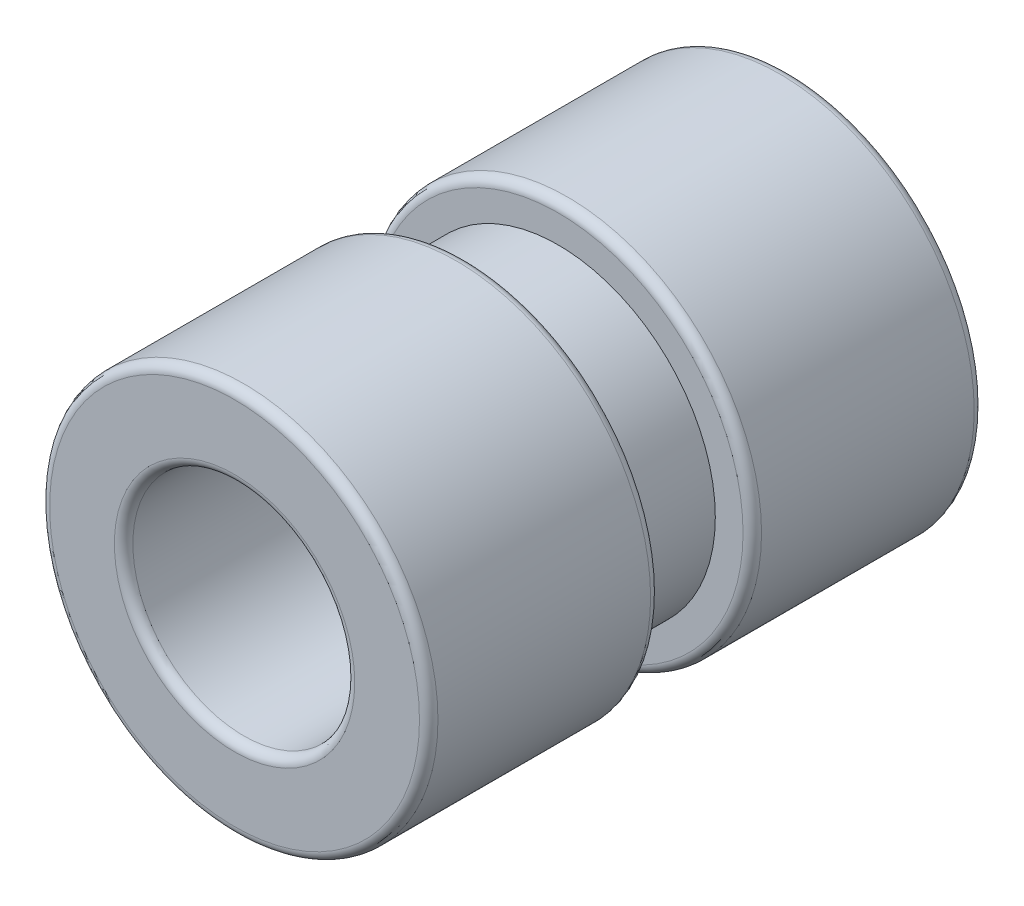
from build123d import *

# Parameters (mm, degrees)
SKETCH1_R           = 10.5
SKETCH1_R_2         = 6
BOSS_EXTRUDE1_DEPTH = 15
SKETCH2_R           = 14.113260249
SKETCH2_R_2         = 8.5
CUT_EXTRUDE1_DEPTH  = 2.5
FILLET1_R           = 0.5


with BuildPart() as part:
    # Sketch1 → Boss-Extrude1 (new, symmetric)
    with BuildSketch(Plane.XY):
        Circle(SKETCH1_R)
        Circle(SKETCH1_R_2, mode=Mode.SUBTRACT)
    extrude(amount=BOSS_EXTRUDE1_DEPTH, both=True)

    # Sketch2 → Cut-Extrude1 (cut, symmetric)
    with BuildSketch(Plane.XY):
        Circle(SKETCH2_R)
        Circle(SKETCH2_R_2, mode=Mode.SUBTRACT)
    extrude(amount=CUT_EXTRUDE1_DEPTH, both=True, mode=Mode.SUBTRACT)

    # Fillet1
    fillet1_edges = [part.edges().sort_by_distance(p)[0] for p in [
        (-10.5, 0, 2.5),
        (-10.5, 0, -2.5),
        (-10.5, 0, -15),
        (-10.5, 0, 15),
        (-6, 0, -15),
        (-6, 0, 15),
    ]]
    fillet(fillet1_edges, radius=FILLET1_R)


solid = part.part
